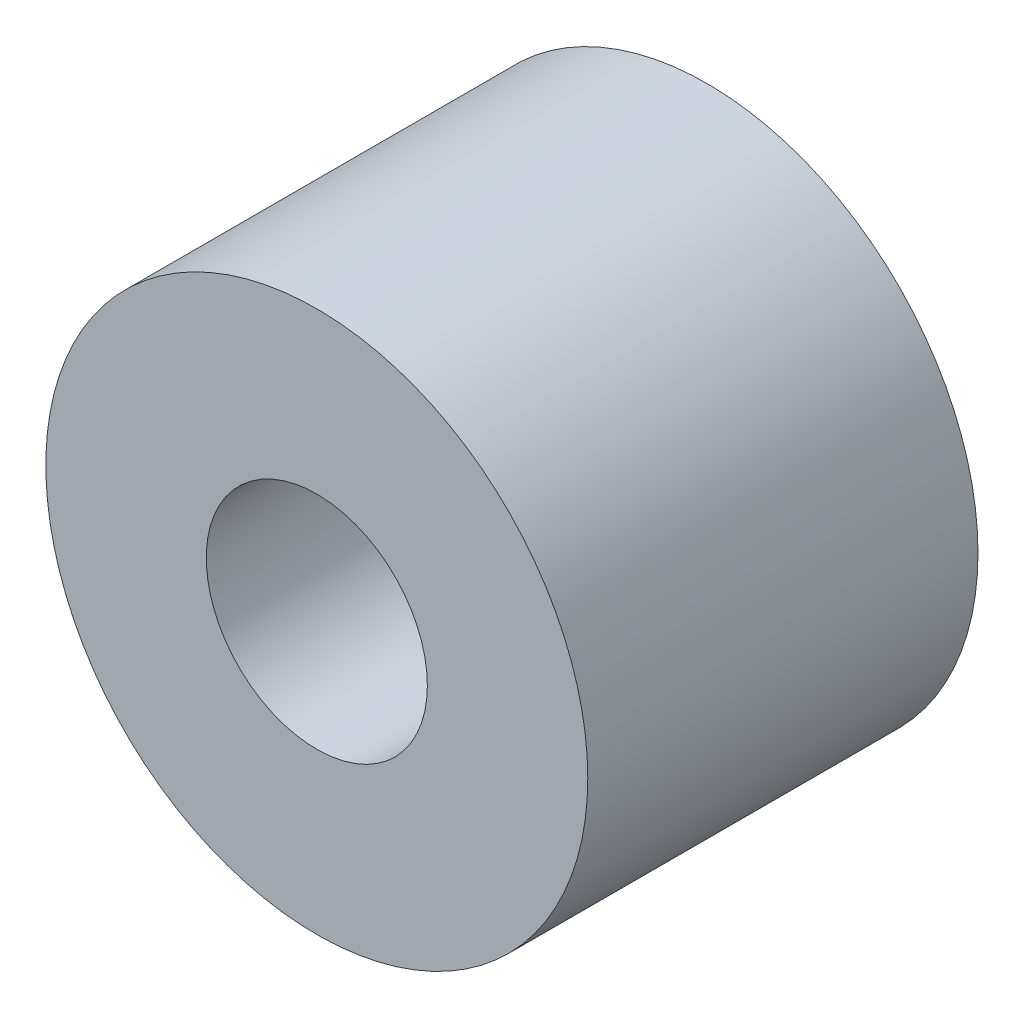
from build123d import *

# Parameters (mm, degrees)
SKETCH1_R              = 12.5
BOSS_EXTRUDE1_DEPTH    = 18
M12_TAPPED_HOLE1_D     = 10.2
M12_TAPPED_HOLE1_DEPTH = 29.25
M12_TAPPED_HOLE1_TIP   = 3.064389157


with BuildPart() as part:
    # Sketch1 → Boss-Extrude1 (new body)
    with BuildSketch(Plane.XY):
        Circle(SKETCH1_R)
    extrude(amount=BOSS_EXTRUDE1_DEPTH)

    # M12 Tapped Hole1
    with Locations(Plane.XY.offset(18)):
        with Locations((0, 0)):
            Hole(M12_TAPPED_HOLE1_D / 2, depth=M12_TAPPED_HOLE1_DEPTH)
            with Locations((0, 0, -(M12_TAPPED_HOLE1_DEPTH + M12_TAPPED_HOLE1_TIP / 2))):  # 118° drill point
                Cone(0, M12_TAPPED_HOLE1_D / 2, M12_TAPPED_HOLE1_TIP, mode=Mode.SUBTRACT)


solid = part.part
